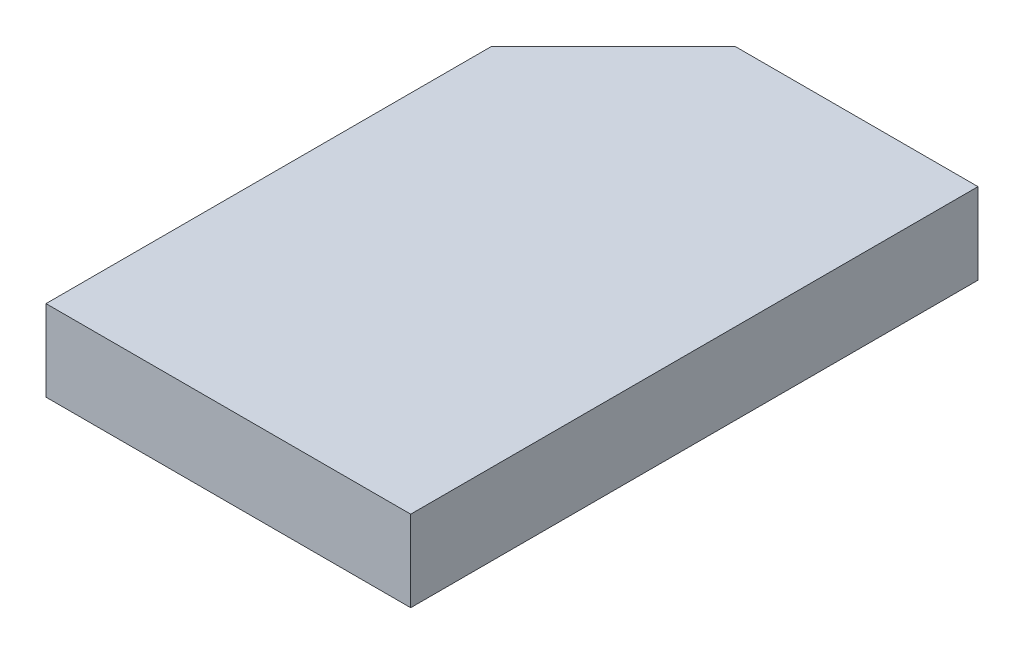
from build123d import *

# Parameters (mm, degrees)
BOSS_EXTRUDE1_DEPTH = 20


with BuildPart() as part:
    # Sketch1 → Boss-Extrude1 (new body)
    with BuildSketch(Plane(origin=(0, 0, 0), x_dir=(1, 0, 0), z_dir=(0, 1, 0))):
        Polygon((-90, 110), (-60, 140), (0, 140), (0, 0), (-90, 0), align=None)
    extrude(amount=BOSS_EXTRUDE1_DEPTH)


solid = part.part
